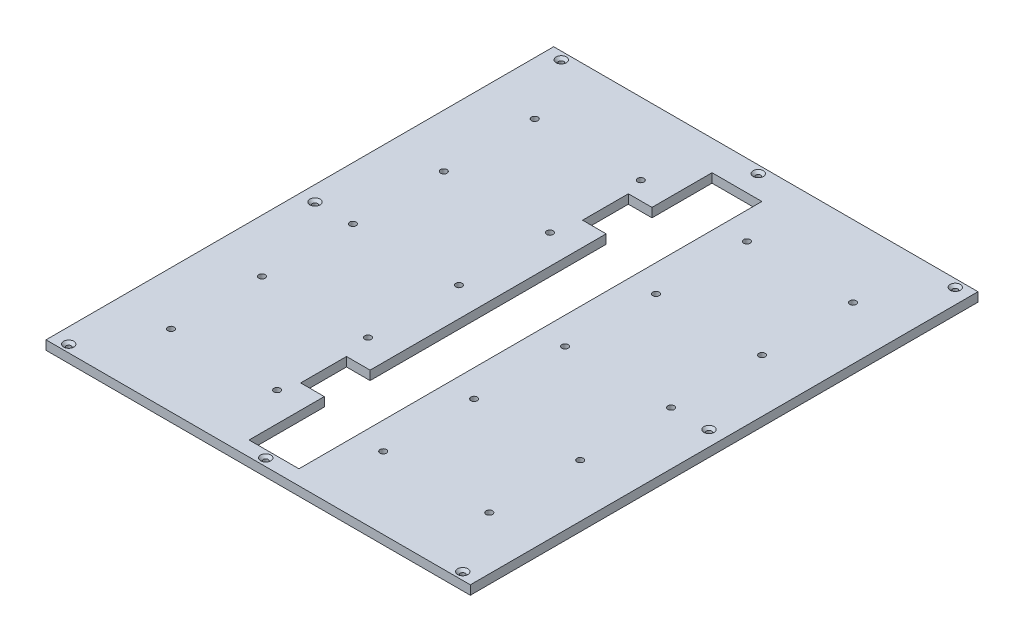
SolidWorks part; units mm, degrees
material "Balsa"
ref_plane "Front Plane" through (0, 0, 0) normal (0, 0, 1) x (1, 0, 0)
ref_plane "Top Plane" through (0, 0, 0) normal (0, 1, 0) x (1, 0, 0)
ref_plane "Right Plane" through (0, 0, 0) normal (1, 0, 0) x (0, 0, -1)
sketch "Sketch1" plane through (0, 0, 0) normal (0, 1, 0) x (1, 0, 0)
  line L1 (-280, 335) -> (280, 335)
  line L2 (-280, 335) -> (-280, -335)
  line L3 (-280, -335) -> (280, -335)
  line L4 (280, 335) -> (280, -335)
  line L5 (-280, 335) -> (280, -335) construction
  line L6 (-280, -335) -> (280, 335) construction
  point P0 (0, 0)
  dimension "D1" = 560
  dimension "D2" = 670
extrude "Boss-Extrude1" add sketch "Sketch1" along normal blind 12
sketch "Sketch3" plane through (0, 12, 0) normal (0, 1, 0) x (1, 0, 0)
  line L0 (-280, -335) -> (280, 335) construction
  line L1 (-280, 335) -> (280, -335) construction
  line L2 (0, 335) -> (0, -335) construction
  line L4 (280, 335) -> (-280, 335) construction
  line L5 (-280, -335) -> (280, -335) construction
  line L6 (280, 0) -> (-280, 0) construction
  line L7 (280, -335) -> (280, 335) construction
  line L8 (-280, 335) -> (-280, -335) construction
  circle A1 centre (210, 240) radius 4.25
  circle A2 centre (70, 240) radius 4.25
  circle A3 centre (210, 120) radius 4.25
  circle A4 centre (70, 120) radius 4.25
  circle A5 centre (70, 0) radius 4.25
  circle A6 centre (210, 0) radius 4.25
  circle A7 centre (0, 0) radius 0.6396
  dimension "D7" = 8.5
  dimension "D3" = 70
  dimension "D4" = 95
  dimension "D6" = 140
  dimension "D8" = 120
extrude "Cut-Extrude1" cut sketch "Sketch3" against normal blind 12
mirror "Mirror1" about plane through (0, 0, 0) normal (1, 0, 0) of "Cut-Extrude1"
mirror "Mirror2" about plane through (0, 0, 0) normal (0, 0, 1) of "Mirror1", "Cut-Extrude1"
sketch "Sketch4" plane through (0, 12, 0) normal (0, 1, 0) x (1, 0, 0)
  line L0 (-280, -335) -> (280, 335) construction
  line L1 (-280, 335) -> (280, -335) construction
hole_wizard "CSK for M6 SFHCS1" positions "Sketch8" profile "Sketch9" countersink size "M6" standard "ANSI Metric" end condition through all
sketch "Sketch8" plane through (0, 12, 0) normal (0, 1, 0) x (1, 0, 0)
  line L0 (-280, -335) -> (280, -335) construction
  line L1 (-280, 335) -> (-280, -335) construction
  line L2 (280, 335) -> (-280, 335) construction
  line L3 (280, -335) -> (280, 335) construction
  circle A0 centre (0, 0) radius 5.6595
  point P0 (0, 0)
  point P3 (260, 0)
  point P5 (0, 325)
  point P7 (260, 325)
  point P9 (0, -325)
  point P11 (-260, 0)
  point P13 (-260, 325)
  point P15 (-260, -325)
  point P17 (260, -325)
  dimension "D1" = 10
  dimension "D2" = 10
  dimension "D3" = 10
  dimension "D4" = 20
  dimension "D5" = 20
  dimension "D6" = 10
  dimension "D7" = 10
  dimension "D8" = 10
  dimension "D9" = 20
  dimension "D10" = 20
  dimension "D11" = 20
  dimension "D12" = 20
sketch "Sketch9" plane through (0, 12, 0) normal (1, 0, 0) x (0, 0, 1)
  line L0 (0, 0) -> (0, 12)
  line L1 (0, 12) -> (3.3, 12)
  line L2 (3.3, 12) -> (3.3, 3.42)
  line L3 (3.3, 3.42) -> (6.72, 0)
  line L5 (6.72, 0) -> (0, 0)
  line L6 (-3.3, 3.42) -> (-6.72, 0) construction
  line L11 (0, -6.35) -> (0, 107.95) construction
  dimension "Thru Hole Dia." = 6.6
  dimension "Thru Hole Depth" = 12
  dimension "Near C'Sink Dia." = 13.44
  dimension "Near C'Sink Angle" = 90
sketch "Sketch10" plane through (0, 12, 0) normal (0, 1, 0) x (1, 0, 0)
  line L0 (-31, 295) -> (-31, 216.2276) construction
  line L1 (-31.5, 295.5) -> (34.3, 295.5)
  line L2 (-31.5, 295.5) -> (-31.5, -315.5)
  line L3 (-31.5, -315.5) -> (34.3, -315.5)
  line L4 (34.3, 295.5) -> (34.3, -315.5)
  line L5 (18.8, 295) -> (-31, 295) construction
  line L6 (33.8, -295) -> (33.8, 295) construction
  line L8 (33.8, -315) -> (-31, -315) construction
  dimension "D1" = 0.5
  dimension "D2" = 0.5
  dimension "D3" = 0.5
  dimension "D4" = 0.5
extrude "Cut-Extrude2" cut sketch "Sketch10" against normal blind 111
sketch "Sketch11" plane through (0, 12, 0) normal (0, 1, 0) x (1, 0, 0)
  line L1 (-31, -155.7724) -> (-62.6631, -155.7724)
  line L2 (-31, -155.7724) -> (-31, -216.2276)
  line L3 (-31, -216.2276) -> (-62.6631, -216.2276)
  line L4 (-62.6631, -155.7724) -> (-62.6631, -216.2276)
extrude "Cut-Extrude3" cut sketch "Sketch11" against normal blind 55
mirror "Mirror3" about plane through (0, 0, 0) normal (0, 0, 1) of "Cut-Extrude3"
